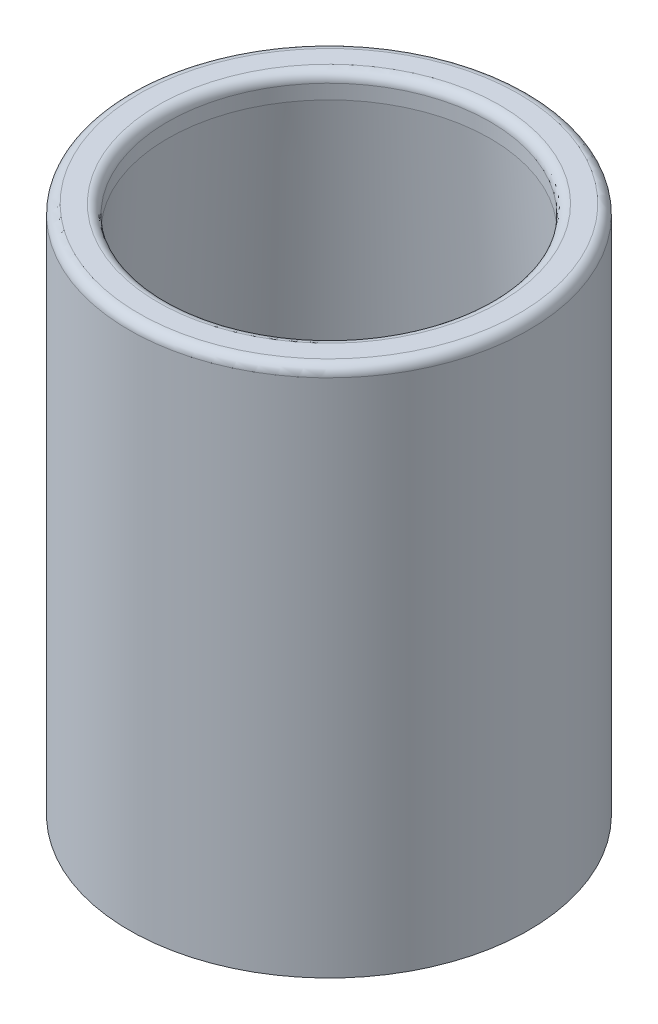
from build123d import *


with BuildPart() as part:
    # Sketch1 → Revolve-Thin1 (revolve)
    with BuildSketch(Plane.XY, mode=Mode.PRIVATE) as revolve_thin1_sk:
        with BuildLine():
            Line((39.5, 110), (35.5, 110))
            ThreePointArc((35.5, 110), (34.085786438, 109.414213562), (33.5, 108))
            Line((33.5, 108), (33.5, 105))
            Line((33.5, 105), (41.5, 0))
            Line((41.5, 0), (41.5, 108))
            ThreePointArc((41.5, 108), (40.914213562, 109.414213562), (39.5, 110))
        make_face()
        with BuildLine():
            Line((39.5, 109), (35.5, 109))
            ThreePointArc((35.5, 109), (34.792893219, 108.707106781), (34.5, 108))
            Line((34.5, 108), (34.5, 105.038040112))
            Line((34.5, 105.038040112), (40.5, 26.288040112))
            Line((40.5, 26.288040112), (40.5, 108))
            ThreePointArc((40.5, 108), (40.207106781, 108.707106781), (39.5, 109))
        make_face(mode=Mode.SUBTRACT)
    revolve(revolve_thin1_sk.sketch.rotate(Axis((0, 0, 0), (0, 1, 0)), 90), axis=Axis((0, 0, 0), (0, 1, 0)))


solid = part.part
